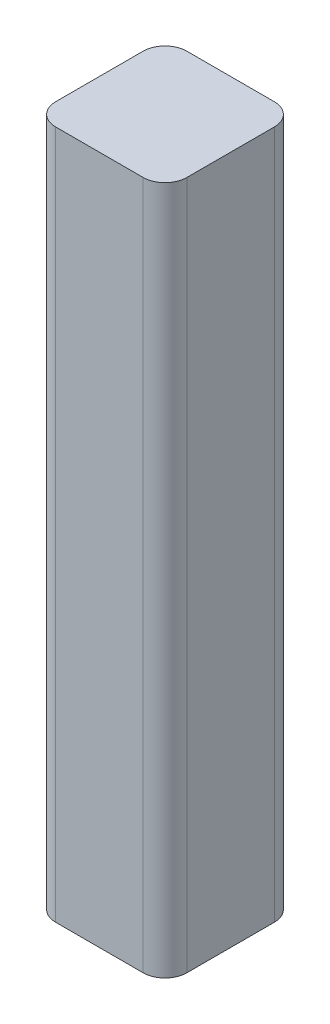
from build123d import *

# Parameters (mm, degrees)
BOSS_EXTRUDE1_DEPTH = 420


with BuildPart() as part:
    # Sketch1 → Boss-Extrude1 (new body)
    with BuildSketch(Plane.XZ):
        with BuildLine():
            Line((40, -26.666666667), (40, 26.666666667))
            ThreePointArc((40, 26.666666667), (36.094757082, 36.094757082), (26.666666667, 40))
            Line((26.666666667, 40), (-26.666666667, 40))
            ThreePointArc((-26.666666667, 40), (-36.094757082, 36.094757082), (-40, 26.666666667))
            Line((-40, 26.666666667), (-40, -26.666666667))
            ThreePointArc((-40, -26.666666667), (-36.094757082, -36.094757082), (-26.666666667, -40))
            Line((-26.666666667, -40), (26.666666667, -40))
            ThreePointArc((26.666666667, -40), (36.094757082, -36.094757082), (40, -26.666666667))
        make_face()
    extrude(amount=-BOSS_EXTRUDE1_DEPTH)


solid = part.part
